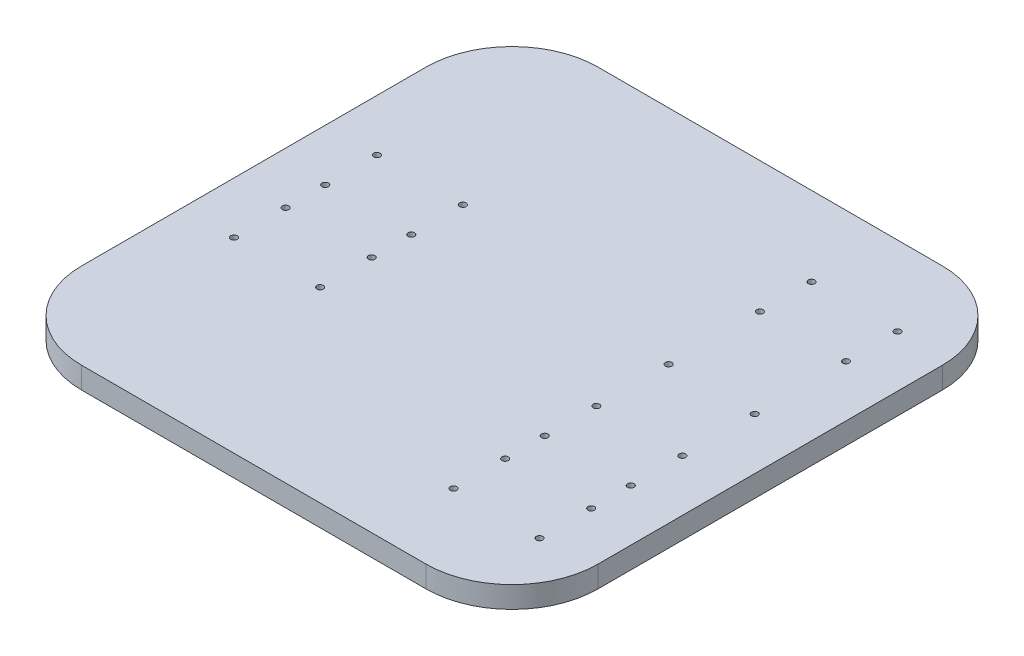
SolidWorks part; units mm, degrees
ref_plane "Front Plane" through (0, 0, 0) normal (0, 0, 1) x (1, 0, 0)
ref_plane "Top Plane" through (0, 0, 0) normal (0, 1, 0) x (1, 0, 0)
ref_plane "Right Plane" through (0, 0, 0) normal (1, 0, 0) x (0, 0, -1)
other "Configuration Table"
sketch "Sketch1" plane through (0, 0, 0) normal (0, 1, 0) x (1, 0, 0)
  line L1 (-40, -60) -> (40, -60)
  line L2 (-60, -40) -> (-60, 40)
  line L3 (-40, 60) -> (40, 60)
  line L4 (60, -40) -> (60, 40)
  line L5 (-60, -60) -> (60, 60) construction
  line L6 (-60, 60) -> (60, -60) construction
  arc A1 (60, 40) -> (40, 60) centre (40, 40) ccw
  arc A3 (40, -60) -> (60, -40) centre (40, -40) ccw
  arc A4 (-40, -60) -> (-60, -40) centre (-40, -40) cw
  arc A5 (-60, 40) -> (-40, 60) centre (-40, 40) cw
  point P0 (0, 0)
  dimension "D1" = 120
  dimension "D2" = 20
  dimension "D3" = 20
  dimension "D4" = 20
extrude "Boss-Extrude1" add sketch "Sketch1" along normal blind 5
sketch "Sketch4" plane through (0, 5, 0) normal (0, 1, 0) x (1, 0, 0)
  line L0 (-37.1419, 0) -> (0, 0) construction
  line L6 (-60, 40) -> (-60, -40) construction
  line L7 (-38, 10.6) -> (-38, 18.2)
  line L12 (-50, 3) -> (-26, 3)
  line L13 (-50, 3) -> (-50, 18.2)
  line L14 (-50, 18.2) -> (-26, 18.2)
  line L15 (-26, 3) -> (-26, 18.2)
  line L16 (-50, 3) -> (-26, 18.2) construction
  line L17 (-50, 18.2) -> (-26, 3) construction
  line L18 (-38, 10.6) -> (-26, 10.6)
  line L19 (-50, -18.2) -> (-26, -3) construction
  line L20 (-50, -3) -> (-26, -18.2) construction
  line L21 (-38, -10.6) -> (-26, -10.6)
  line L22 (-26, -3) -> (-26, -18.2)
  line L23 (-50, -18.2) -> (-26, -18.2)
  line L24 (-50, -3) -> (-50, -18.2)
  line L25 (-50, -3) -> (-26, -3)
  line L26 (-38, -10.6) -> (-38, -18.2)
  line L27 (60, 0) -> (60, 25)
  line L28 (60, -40) -> (60, 40) construction
  line L29 (60, 25) -> (0, 25) construction
  line L30 (38, 35.6) -> (38, 43.2)
  line L31 (26, 28) -> (50, 28)
  line L32 (26, 28) -> (26, 43.2)
  line L33 (26, 43.2) -> (50, 43.2)
  line L34 (50, 28) -> (50, 43.2)
  line L35 (26, 28) -> (50, 43.2) construction
  line L36 (26, 43.2) -> (50, 28) construction
  line L37 (38, 35.6) -> (50, 35.6)
  line L38 (26, 6.8) -> (50, 22) construction
  line L39 (26, 22) -> (50, 6.8) construction
  line L40 (38, 14.4) -> (50, 14.4)
  line L45 (50, 22) -> (50, 6.8)
  line L46 (26, 6.8) -> (50, 6.8)
  line L47 (26, 22) -> (26, 6.8)
  line L48 (26, 22) -> (50, 22)
  line L49 (38, 14.4) -> (38, 6.8)
  line L50 (26, -22) -> (50, -6.8) construction
  line L51 (26, -6.8) -> (50, -22) construction
  line L52 (26, -43.2) -> (50, -28) construction
  line L53 (26, -28) -> (50, -43.2) construction
  line L54 (38, -14.4) -> (38, -6.8)
  line L55 (26, -22) -> (50, -22)
  line L56 (26, -22) -> (26, -6.8)
  line L57 (26, -6.8) -> (50, -6.8)
  line L58 (50, -22) -> (50, -6.8)
  line L59 (38, -14.4) -> (50, -14.4)
  line L60 (38, -35.6) -> (50, -35.6)
  line L61 (50, -28) -> (50, -43.2)
  line L62 (26, -43.2) -> (50, -43.2)
  line L63 (26, -28) -> (26, -43.2)
  line L64 (26, -28) -> (50, -28)
  line L65 (38, -35.6) -> (38, -43.2)
  circle A1 centre (-48, 16.6) radius 0.75
  circle A2 centre (-28, 16.6) radius 0.75
  circle A3 centre (-48, 4.6) radius 0.75
  circle A4 centre (-28, 4.6) radius 0.75
  circle A5 centre (-28, -4.6) radius 0.75
  circle A6 centre (-48, -4.6) radius 0.75
  circle A7 centre (-28, -16.6) radius 0.75
  circle A8 centre (-48, -16.6) radius 0.75
  circle A9 centre (28, 41.6) radius 0.75
  circle A10 centre (48, 41.6) radius 0.75
  circle A11 centre (28, 29.6) radius 0.75
  circle A12 centre (48, 29.6) radius 0.75
  circle A17 centre (48, 20.4) radius 0.75
  circle A18 centre (28, 20.4) radius 0.75
  circle A19 centre (48, 8.4) radius 0.75
  circle A20 centre (28, 8.4) radius 0.75
  circle A21 centre (28, -8.4) radius 0.75
  circle A22 centre (48, -8.4) radius 0.75
  circle A23 centre (28, -20.4) radius 0.75
  circle A24 centre (48, -20.4) radius 0.75
  circle A25 centre (48, -29.6) radius 0.75
  circle A26 centre (28, -29.6) radius 0.75
  circle A27 centre (48, -41.6) radius 0.75
  circle A28 centre (28, -41.6) radius 0.75
  point P8 (-38, 10.6)
  point P36 (-38, -10.6)
  point P45 (38, 35.6)
  point P73 (38, 14.4)
  point P105 (38, -14.4)
  point P106 (38, -35.6)
  dimension "D6" = 10
  dimension "D7" = 1.5
  dimension "D8" = 25
  dimension "D5" = 6
  dimension "D14" = 1.5
  dimension "D2" = 15.2
  dimension "D3" = 3
  dimension "D4" = 10
  dimension "D9" = 24
  dimension "D10" = 24
  dimension "D11" = 15.2
  dimension "D12" = 6
  dimension "D13" = 10
  dimension "D15" = 10
  dimension "D16" = 3
extrude "Cut-Extrude1" cut sketch "Sketch4" against normal through all contours A1 | A3 | A4 | A2 | A6 | A8 | A7 | A5 | A21 | A22 | A23 | A24 | A25 | A26 | A28 | A27 | A20 | A19 | A11 | A12 | A9 | A10
